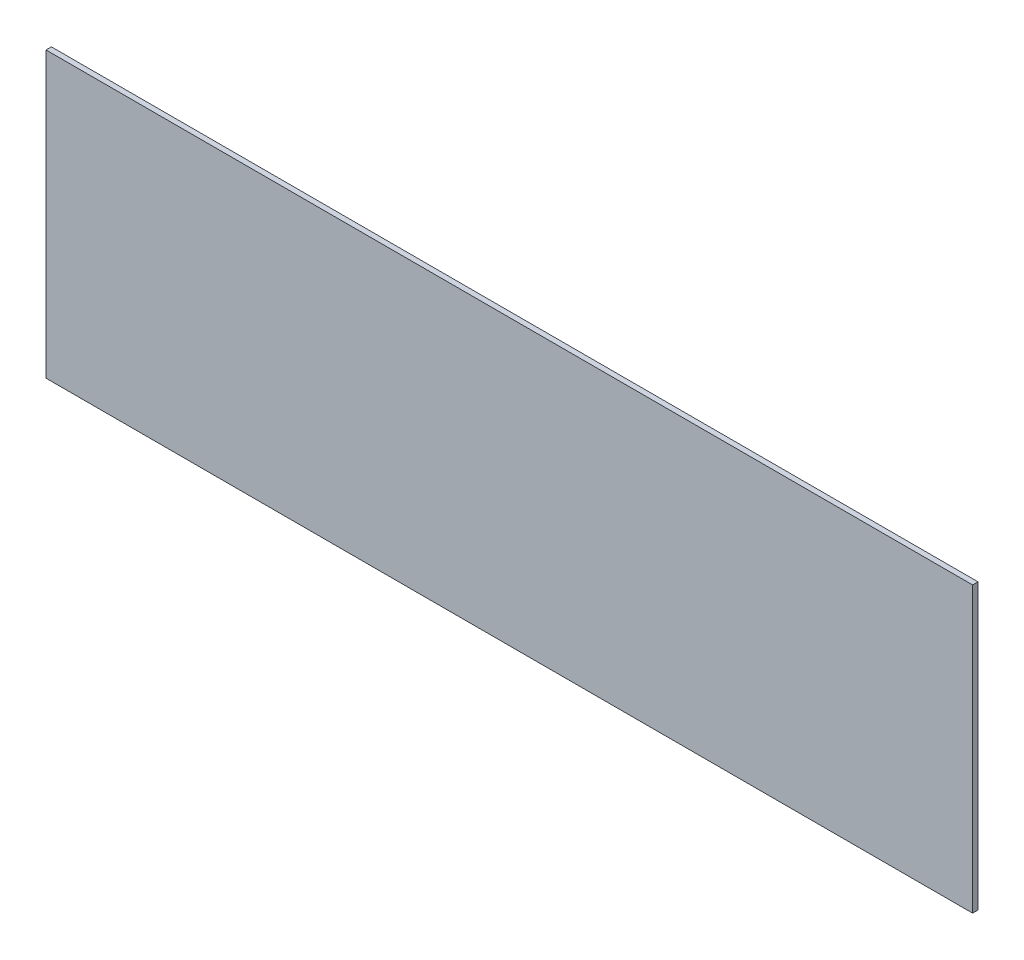
SolidWorks part; units mm, degrees
ref_plane "Frontal" through (0, 0, 0) normal (0, 0, 1) x (1, 0, 0)
ref_plane "Superior" through (0, 0, 0) normal (0, 1, 0) x (1, 0, 0)
ref_plane "Direito" through (0, 0, 0) normal (1, 0, 0) x (0, 0, -1)
sketch "Sketch1" plane through (0, 0, 0) normal (0, 0, 1) x (1, 0, 0)
  line L1 (-257.5, 79) -> (257.5, 79)
  line L2 (-257.5, 79) -> (-257.5, -79)
  line L3 (-257.5, -79) -> (257.5, -79)
  line L4 (257.5, 79) -> (257.5, -79)
  line L5 (-257.5, 79) -> (257.5, -79) construction
  line L6 (-257.5, -79) -> (257.5, 79) construction
  point P0 (0, 0)
  dimension "D1" = 158
  dimension "D2" = 515
extrude "Boss-Extrude1" add sketch "Sketch1" along normal blind 3
